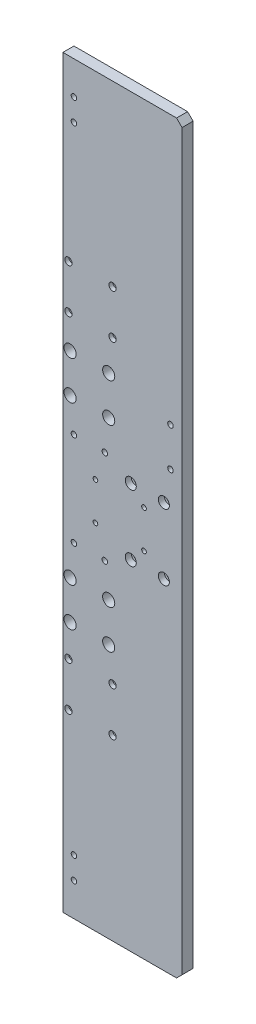
SolidWorks part; units mm, degrees
material "6061-T6"
ref_plane "前视基准面" through (0, 0, 0) normal (0, 0, 1) x (1, 0, 0)
ref_plane "上视基准面" through (0, 0, 0) normal (0, 1, 0) x (1, 0, 0)
ref_plane "右视基准面" through (0, 0, 0) normal (1, 0, 0) x (0, 0, -1)
sketch "草图1" plane through (0, 0, 0) normal (0, 0, 1) x (1, 0, 0)
  line L1 (108, 675) -> (0, 675)
  line L2 (108, 675) -> (108, 0)
  line L3 (108, 0) -> (0, 0)
  line L4 (0, 675) -> (0, 0)
  dimension "D1" = 675
  dimension "D2" = 108
extrude "凸台-拉伸1" add sketch "草图1" along normal blind 10
hole_wizard "M6 螺纹孔1" positions "草图2" profile "草图3" tap size "M6" standard "ISO" end condition through all
sketch "草图2" plane through (0, 0, 10) normal (0, 0, 1) x (1, 0, 0)
  line L0 (0, 337.5) -> (151.089, 337.5) construction
  line L1 (0, 675) -> (0, 0) construction
  line L3 (10, 30) -> (10, 50) construction
  line L5 (0, 0) -> (108, 0) construction
  point P0 (10, 645)
  point P2 (10, 625)
  point P13 (10, 50)
  point P14 (10, 30)
  dimension "D1" = 10
  dimension "D2" = 20
  dimension "D3" = 30
sketch "草图3" plane through (10, 645, 10) normal (1, 0, 0) x (0, -1, 0)
  line L0 (0, 0) -> (0, 10)
  line L1 (0, 10) -> (2.5, 10)
  line L2 (2.5, 10) -> (2.5, 0)
  line L5 (2.5, 0) -> (0, 0)
  line L11 (0, -6.35) -> (0, 107.95) construction
  dimension "通孔螺纹孔钻头直径" = 5
  dimension "通孔螺纹孔钻头深度" = 10
cosmetic thread "孔螺蚊线1" parameters "D2"=6
cosmetic thread "孔螺蚊线2" parameters "D2"=6
cosmetic thread "孔螺蚊线3" parameters "D2"=6
cosmetic thread "孔螺蚊线4" parameters "D2"=6
hole_wizard "M6 六角凹头螺钉的柱形沉头孔1" positions "草图4" profile "草图5" counterbore size "M6" standard "ISO" end condition through all
sketch "草图4" plane through (0, 0, 0) normal (0, 0, -1) x (-1, 0, 0)
  line L0 (0, 337.5) -> (27.2492, 337.5) construction
  line L1 (0, 675) -> (0, 0) construction
  line L3 (-45, 161.5) -> (-5, 161.5) construction
  line L4 (-5, 161.5) -> (-5, 201.5) construction
  line L5 (-5, 201.5) -> (-45, 201.5) construction
  line L6 (-45, 201.5) -> (-45, 161.5) construction
  line L8 (-5, 201.5) -> (-5, 473.5) construction
  line L9 (-5, 473.5) -> (-5, 513.5) construction
  line L10 (-5, 513.5) -> (-45, 513.5) construction
  line L11 (-45, 513.5) -> (-45, 473.5) construction
  line L12 (-45, 473.5) -> (-5, 473.5) construction
  point P0 (-45, 513.5)
  point P2 (-5, 513.5)
  point P4 (-45, 473.5)
  point P6 (-5, 473.5)
  point P15 (-5, 201.5)
  point P16 (-45, 201.5)
  point P17 (-5, 161.5)
  point P18 (-45, 161.5)
  point P37 (-5, 181.5)
  dimension "D1" = 272
  dimension "D2" = 5
  dimension "D3" = 40
  dimension "D4" = 40
sketch "草图5" plane through (45, 513.5, 0) normal (1, 0, 0) x (0, 1, 0)
  line L0 (0, 0) -> (0, 10)
  line L1 (0, 10) -> (3.3, 10)
  line L3 (3.3, 10) -> (3.3, 6.4)
  line L4 (3.3, 6.4) -> (5.5, 6.4)
  line L5 (5.5, 6.4) -> (5.5, 0)
  line L7 (5.5, 0) -> (0, 0)
  line L11 (0, -6.35) -> (0, 107.95) construction
  dimension "通孔孔直径" = 6.6
  dimension "通孔孔深度" = 10
  dimension "柱形沉头孔直径" = 11
  dimension "柱形沉头孔深度" = 6.4
hole_wizard "M5 螺纹孔1" positions "草图6" profile "草图7" tap size "M5" standard "ISO"
sketch "草图6" plane through (0, 0, 10) normal (0, 0, 1) x (1, 0, 0)
  line L0 (29.5, 320.5) -> (73.5, 320.5) construction
  line L1 (73.5, 320.5) -> (73.5, 354.5) construction
  line L2 (73.5, 354.5) -> (29.5, 354.5) construction
  line L3 (29.5, 354.5) -> (29.5, 320.5) construction
  line L5 (29.5, 337.5) -> (0, 337.5) construction
  line L6 (0, 675) -> (0, 0) construction
  point P0 (29.5, 354.5)
  point P2 (73.5, 354.5)
  point P4 (29.5, 320.5)
  point P6 (73.5, 320.5)
  dimension "D1" = 29.5
  dimension "D2" = 44
  dimension "D3" = 34
sketch "草图7" plane through (29.5, 354.5, 10) normal (1, 0, 0) x (0, -1, 0)
  line L0 (0, 0) -> (0, 15.2618)
  line L1 (0, 15.2618) -> (2.1, 14)
  line L2 (2.1, 14) -> (2.1, 0)
  line L5 (2.1, 0) -> (0, 0)
  line L10 (0, 15.2618) -> (-2.1, 14) construction
  line L11 (0, -6.35) -> (0, 107.95) construction
  dimension "螺纹孔钻头直径" = 4.2
  dimension "螺纹孔钻头深度" = 14
  dimension "导头角度" = 118
cosmetic thread "孔螺蚊线5" parameters "D1"=10, "D2"=5
cosmetic thread "孔螺蚊线6" parameters "D1"=10, "D2"=5
cosmetic thread "孔螺蚊线7" parameters "D1"=10, "D2"=5
cosmetic thread "孔螺蚊线8" parameters "D1"=10, "D2"=5
hole_wizard "M6 螺纹孔2" positions "草图8" profile "草图9" tap size "M6" standard "ISO"
sketch "草图8" plane through (0, 0, 10) normal (0, 0, 1) x (1, 0, 0)
  line L0 (97.5, 396.5) -> (97.5, 431.5) construction
  line L2 (108, 0) -> (108, 675) construction
  line L3 (108, 337.5) -> (132.6323, 337.5) construction
  point P0 (97.5, 431.5)
  point P2 (97.5, 396.5)
  dimension "D1" = 10.5
  dimension "D2" = 35
  dimension "D3" = 59
sketch "草图9" plane through (97.5, 431.5, 10) normal (1, 0, 0) x (0, -1, 0)
  line L0 (0, 0) -> (0, 18.5022)
  line L1 (0, 18.5022) -> (2.5, 17)
  line L2 (2.5, 17) -> (2.5, 0)
  line L5 (2.5, 0) -> (0, 0)
  line L10 (0, 18.5022) -> (-2.5, 17) construction
  line L11 (0, -6.35) -> (0, 107.95) construction
  dimension "螺纹孔钻头直径" = 5
  dimension "螺纹孔钻头深度" = 17
  dimension "导头角度" = 118
cosmetic thread "孔螺蚊线9" parameters "D1"=10, "D2"=6
cosmetic thread "孔螺蚊线10" parameters "D1"=10, "D2"=6
hole_wizard "M5 六角凹头螺钉的柱形沉头孔1" positions "草图10" profile "草图11" counterbore size "M5" standard "ISO"
sketch "草图10" plane through (0, 0, 10) normal (0, 0, 1) x (1, 0, 0)
  line L0 (91.5, 367.5) -> (61.5, 367.5) construction
  line L1 (61.5, 367.5) -> (61.5, 307.5) construction
  line L2 (61.5, 307.5) -> (91.5, 307.5) construction
  line L3 (91.5, 307.5) -> (91.5, 367.5) construction
  line L5 (91.5, 337.5) -> (108, 337.5) construction
  line L6 (108, 0) -> (108, 675) construction
  point P0 (61.5, 367.5)
  point P2 (91.5, 367.5)
  point P4 (61.5, 307.5)
  point P6 (91.5, 307.5)
  dimension "D1" = 16.5
  dimension "D2" = 30
  dimension "D3" = 60
sketch "草图11" plane through (61.5, 367.5, 10) normal (1, 0, 0) x (0, -1, 0)
  line L0 (0, 0) -> (0, 15.6524)
  line L1 (0, 15.6524) -> (2.75, 14)
  line L2 (2.75, 14) -> (2.75, 5.4)
  line L3 (2.75, 5.4) -> (5, 5.4)
  line L4 (5, 5.4) -> (5, 0)
  line L5 (5, 0) -> (0, 0)
  line L10 (0, 15.6524) -> (-2.75, 14) construction
  line L11 (0, -6.35) -> (0, 107.95) construction
  dimension "孔直径" = 5.5
  dimension "孔深度" = 14
  dimension "柱形沉头孔直径" = 10
  dimension "柱形沉头孔深度" = 5.4
  dimension "导头角度" = 118
hole_wizard "M6 螺纹孔3" positions "草图12" profile "草图13" tap size "M6" standard "ISO"
sketch "草图12" plane through (0, 0, 0) normal (0, 0, -1) x (-1, 0, 0)
  line L0 (-38, 295) -> (-10, 295) construction
  line L1 (-10, 295) -> (-10, 380) construction
  line L2 (-10, 380) -> (-38, 380) construction
  line L3 (-38, 380) -> (-38, 295) construction
  line L7 (-45, 473.5) -> (-45, 201.5) construction
  line L10 (0, 471.2087) -> (0, 203.7913) construction
  line L11 (-38, 337.5) -> (-45, 337.5) construction
  point P0 (-38, 380)
  point P2 (-10, 380)
  point P4 (-38, 295)
  point P6 (-10, 295)
  dimension "D2" = 85
  dimension "D3" = 28
  dimension "D4" = 10
sketch "草图13" plane through (38, 380, 0) normal (1, 0, 0) x (0, 1, 0)
  line L0 (0, 0) -> (0, 18.5022)
  line L1 (0, 18.5022) -> (2.5, 17)
  line L2 (2.5, 17) -> (2.5, 0)
  line L5 (2.5, 0) -> (0, 0)
  line L10 (0, 18.5022) -> (-2.5, 17) construction
  line L11 (0, -6.35) -> (0, 107.95) construction
  dimension "螺纹孔钻头直径" = 5
  dimension "螺纹孔钻头深度" = 17
  dimension "导头角度" = 118
cosmetic thread "孔螺蚊线11" parameters "D1"=10, "D2"=6
cosmetic thread "孔螺蚊线12" parameters "D1"=10, "D2"=6
cosmetic thread "孔螺蚊线13" parameters "D1"=10, "D2"=6
cosmetic thread "孔螺蚊线14" parameters "D1"=10, "D2"=6
sketch "草图14" plane through (0, 0, 10) normal (0, 0, 1) x (1, 0, 0)
  line L0 (6.5, 231) -> (41.5, 231) construction
  line L1 (41.5, 231) -> (41.5, 266) construction
  line L2 (41.5, 266) -> (6.5, 266) construction
  line L3 (6.5, 266) -> (6.5, 409) construction
  line L4 (6.5, 409) -> (41.5, 409) construction
  line L5 (41.5, 409) -> (41.5, 444) construction
  line L6 (41.5, 444) -> (6.5, 444) construction
  line L7 (6.5, 444) -> (6.5, 409) construction
  line L8 (41.5, 266) -> (41.5, 409) construction
  line L9 (6.5, 266) -> (6.5, 231) construction
  line L10 (6.5, 337.5) -> (0, 337.5) construction
  line L11 (0, 675) -> (0, 0) construction
  circle A0 centre (41.5, 444) radius 5.5
  circle A1 centre (6.5, 444) radius 5.5
  circle A2 centre (41.5, 409) radius 5.5
  circle A3 centre (6.5, 409) radius 5.5
  circle A4 centre (41.5, 266) radius 5.5
  circle A5 centre (41.5, 231) radius 5.5
  circle A6 centre (6.5, 231) radius 5.5
  circle A7 centre (6.5, 266) radius 5.5
  dimension "D6" = 11
  dimension "D1" = 35
  dimension "D2" = 35
  dimension "D3" = 143
  dimension "D4" = 35
  dimension "D5" = 6.5
extrude "切除-拉伸1" cut sketch "草图14" against normal blind 60
chamfer "倒角1" distance 5 angle 45 2 edges at (108, 0, 5) (108, 675, 5)
